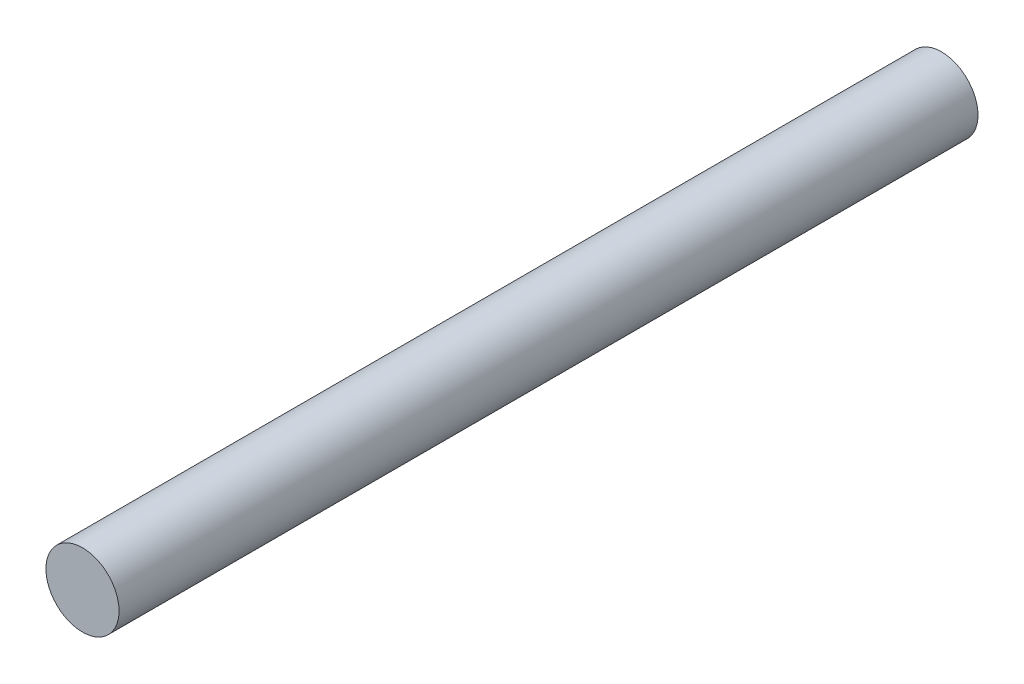
from build123d import *

# Parameters (mm, degrees)
SKETCH_1_R      = 2
EXTRUDE_1_DEPTH = 47


with BuildPart() as part:
    # 草图1 → 凸台-拉伸1 (new body)
    with BuildSketch(Plane.XY):
        Circle(SKETCH_1_R)
    extrude(amount=EXTRUDE_1_DEPTH)


solid = part.part
